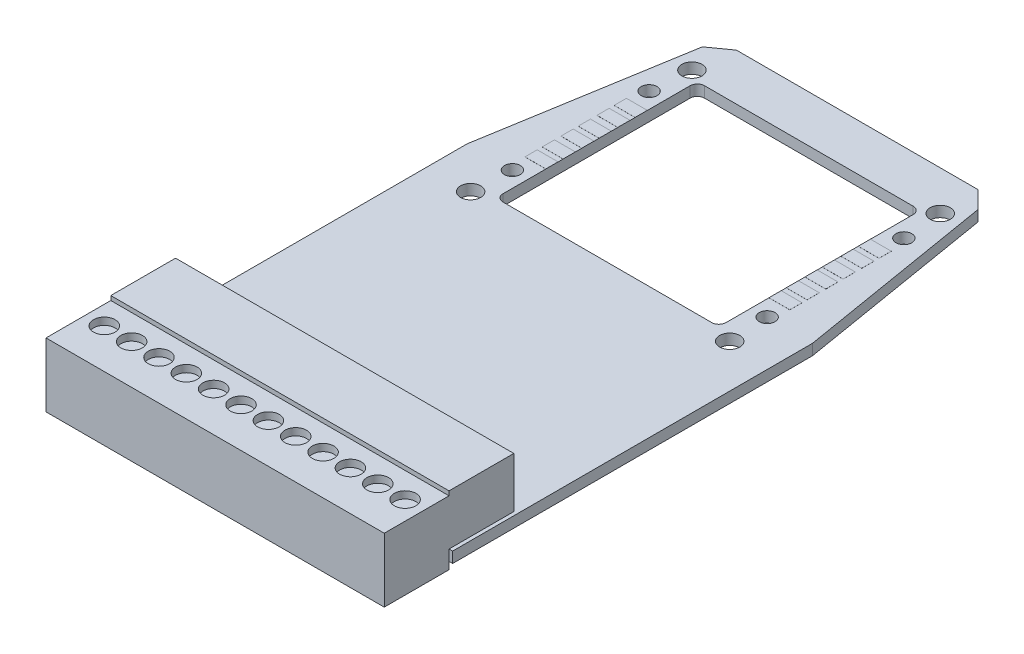
from build123d import *
from OCP.BRepFilletAPI import BRepFilletAPI_MakeChamfer

# Parameters (mm, degrees)
SKETCH1_W                  = 48
SKETCH1_H                  = 80
BOSS_EXTRUDE1_DEPTH        = 0.75
CUT_EXTRUDE1_DEPTH         = 47.671725916
SKETCH3_W                  = 31
SKETCH3_H                  = 28
CUT_EXTRUDE2_DEPTH         = 47.671725916
FILLET1_R                  = 1
F_2_8_2_8_DIAMETER_HOLE1_D = 2.8
F_2_2_2_2_DIAMETER_HOLE1_D = 2.2
SKETCH8_W                  = 47
SKETCH8_H                  = 9
BOSS_EXTRUDE2_DEPTH        = 7
SKETCH9_W                  = 47
SKETCH9_H                  = 8.9
BOSS_EXTRUDE3_DEPTH        = 9
SKETCH10_R                 = 1.5
CUT_EXTRUDE3_DEPTH         = 1
LPATTERN1_COUNT            = 12
LPATTERN1_PITCH            = 3.8
SKETCH11_W                 = 2.9
SKETCH11_H                 = 1.7
BOSS_EXTRUDE4_DEPTH        = 0.01
LPATTERN2_COUNT            = 3
LPATTERN2_PITCH            = 5
CHAMFER1_SIZE              = 2
CHAMFER1_SIZE2             = 2.433105012


with BuildPart() as part:
    # Sketch1 → Boss-Extrude1 (new, symmetric)
    with BuildSketch(Plane(origin=(0, 0, 0), x_dir=(1, 0, 0), z_dir=(0, 1, 0))):
        Rectangle(SKETCH1_W, SKETCH1_H)
    extrude(amount=BOSS_EXTRUDE1_DEPTH, both=True)

    # Sketch2 → Cut-Extrude1 (cut, through all)
    with BuildSketch(Plane(origin=(0, 0.75, 0), x_dir=(1, 0, 0), z_dir=(0, 1, 0))):
        Polygon((-19, 40), (-24, 40), (-24, 10), align=None)
        Polygon((19, 40), (24, 40), (24, 10), align=None)
    extrude(amount=-CUT_EXTRUDE1_DEPTH, mode=Mode.SUBTRACT)

    # Sketch3 → Cut-Extrude2 (cut, through all)
    with BuildSketch(Plane(origin=(0, 0.75, 0), x_dir=(1, 0, 0), z_dir=(0, 1, 0))):
        with Locations((0, 19.5)):
            Rectangle(SKETCH3_W, SKETCH3_H)
    extrude(amount=-CUT_EXTRUDE2_DEPTH, mode=Mode.SUBTRACT)

    # Fillet1
    fillet1_edges = [part.edges().sort_by_distance(p)[0] for p in [
        (15.5, 0, -33.5),
        (15.5, 0, -5.5),
        (-15.5, 0, -5.5),
        (-15.5, 0, -33.5),
    ]]
    fillet(fillet1_edges, radius=FILLET1_R)

    # Ø2.8 (2.8) Diameter Hole1 (through all)
    with Locations(Plane(origin=(0, 0.75, 0), x_dir=(1, 0, 0), z_dir=(0, 1, 0))):
        with Locations((17.25, 34.5), (18, 4.5), (-17.25, 34.5), (-18, 4.5)):
            Hole(F_2_8_2_8_DIAMETER_HOLE1_D / 2)

    # Ø2.2 (2.2) Diameter Hole1 (through all)
    with Locations(Plane(origin=(0, 0.75, 0), x_dir=(1, 0, 0), z_dir=(0, 1, 0))):
        with Locations((17.7, 29), (17.7, 10), (-17.7, 10), (-17.7, 29)):
            Hole(F_2_2_2_2_DIAMETER_HOLE1_D / 2)

    # Sketch8 → Boss-Extrude2 (add)
    with BuildSketch(Plane(origin=(0, 0.75, 0), x_dir=(1, 0, 0), z_dir=(0, 1, 0))):
        with Locations((0, -35.5)):
            Rectangle(SKETCH8_W, SKETCH8_H)
    extrude(amount=BOSS_EXTRUDE2_DEPTH)

    # Sketch9 → Boss-Extrude3 (add)
    with BuildSketch(Plane.XY.offset(40)):
        with Locations((0, 2.7)):
            Rectangle(SKETCH9_W, SKETCH9_H)
    extrude(amount=BOSS_EXTRUDE3_DEPTH)

    # Sketch10 → Cut-Extrude3 (cut)
    with BuildSketch(Plane(origin=(0, 7.15, 0), x_dir=(1, 0, 0), z_dir=(0, 1, 0))):
        with Locations(Location((-20.9, -43.5, 0), (0, 0, 270))):
            Circle(SKETCH10_R)
    cut_extrude3 = extrude(amount=-CUT_EXTRUDE3_DEPTH, mode=Mode.SUBTRACT)

    # LPattern1: Cut-Extrude3 ×12
    with Locations(*[(i * LPATTERN1_PITCH, 0, 0) for i in range(1, LPATTERN1_COUNT)]):
        add(cut_extrude3, mode=Mode.SUBTRACT)

    # Sketch11 → Boss-Extrude4 (add)
    with BuildSketch(Plane(origin=(0, 0.75, 0), x_dir=(1, 0, 0), z_dir=(0, 1, 0))):
        with Locations((-16.95, 23.3)):
            Rectangle(SKETCH11_W, SKETCH11_H)
        with Locations((16.95, 25.7)):
            Rectangle(SKETCH11_W, SKETCH11_H)
        with Locations((-16.95, 25.7)):
            Rectangle(SKETCH11_W, SKETCH11_H)
        with Locations((16.95, 23.3)):
            Rectangle(SKETCH11_W, SKETCH11_H)
    boss_extrude4 = extrude(amount=BOSS_EXTRUDE4_DEPTH)

    # LPattern2: Boss-Extrude4 ×3
    with Locations(*[(0, 0, i * LPATTERN2_PITCH) for i in range(1, LPATTERN2_COUNT)]):
        add(boss_extrude4)

    # Chamfer1: one chamfer whose edges measure the first distance from different faces: ONE call of the kernel's chamfer builder (chamfer() names one face for all edges)
    chamfer1_edges_1 = [part.edges().sort_by_distance(p)[0] for p in [
        (-19, 0, -40),
    ]]
    chamfer1_side_1 = [part.faces().sort_by_distance(p)[0] for p in [
        (-21.5, 0, -25),
    ]]
    chamfer1_edges_2 = [part.edges().sort_by_distance(p)[0] for p in [
        (19, 0, -40),
    ]]
    chamfer1_side_2 = [part.faces().sort_by_distance(p)[0] for p in [
        (0, 0, -40),
    ]]
    chamfer1 = BRepFilletAPI_MakeChamfer(part.part.solid().wrapped)
    for e in chamfer1_edges_1:
        chamfer1.Add(CHAMFER1_SIZE, CHAMFER1_SIZE2, e.wrapped, chamfer1_side_1[0].wrapped)  # the first distance lies on this face
    for e in chamfer1_edges_2:
        chamfer1.Add(CHAMFER1_SIZE, CHAMFER1_SIZE2, e.wrapped, chamfer1_side_2[0].wrapped)  # the first distance lies on this face
    add(Compound.cast(chamfer1.Shape()), mode=Mode.REPLACE)


solid = part.part
